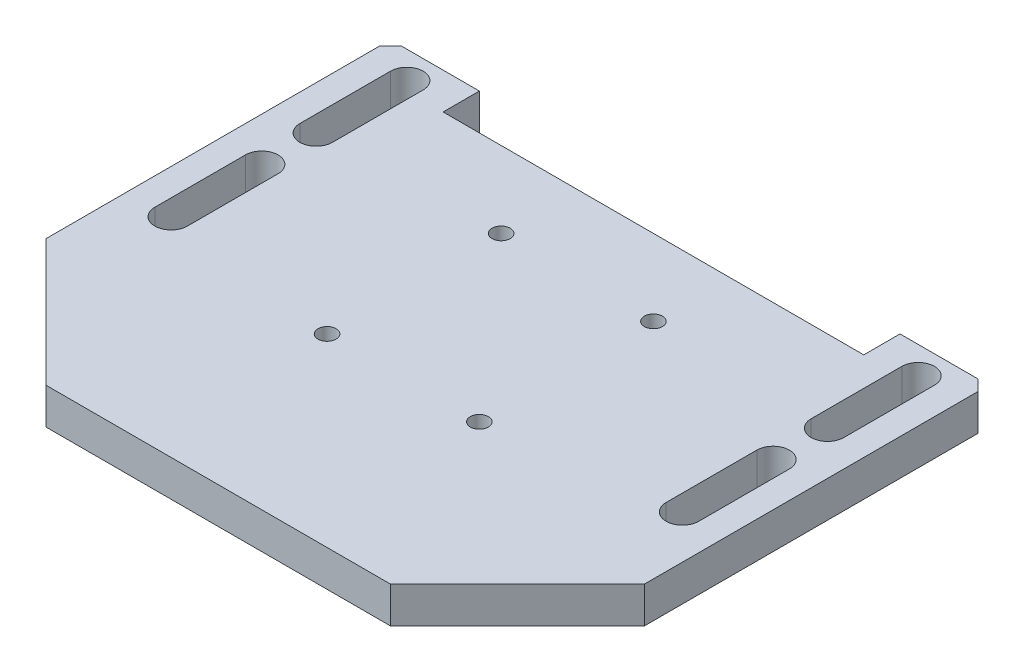
SolidWorks part; units mm, degrees
ref_plane "前视基准面" through (0, 0, 0) normal (0, 0, 1) x (1, 0, 0)
ref_plane "上视基准面" through (0, 0, 0) normal (0, 1, 0) x (1, 0, 0)
ref_plane "右视基准面" through (0, 0, 0) normal (1, 0, 0) x (0, 0, -1)
sketch "草图2" plane through (0, 0, 0) normal (0, 1, 0) x (1, 0, 0)
  line L1 (-82.5, 65) -> (82.5, 65)
  line L2 (-82.5, 65) -> (-82.5, -65)
  line L3 (-82.5, -65) -> (82.5, -65)
  line L4 (82.5, 65) -> (82.5, -65)
  line L5 (-82.5, 65) -> (82.5, -65) construction
  line L6 (-82.5, -65) -> (82.5, 65) construction
  point P0 (0, 0)
  dimension "D1" = 165
  dimension "D2" = 130
extrude "凸台-拉伸1" add sketch "草图2" along normal blind 10
sketch "草图3" plane through (0, 10, 0) normal (0, 1, 0) x (1, 0, 0)
  line L0 (82.5, 65) -> (-82.5, 65) construction
  line L1 (-58, 65) -> (58, 65)
  line L2 (-58, 65) -> (-58, 55)
  line L3 (-58, 55) -> (58, 55)
  line L4 (58, 65) -> (58, 55)
  line L5 (0, 0) -> (0, 72.8477) construction
  dimension "D1" = 116
  dimension "D2" = 10
extrude "切除-拉伸1" cut sketch "草图3" against normal blind 10
sketch "草图4" plane through (0, 10, 0) normal (0, 1, 0) x (1, 0, 0)
  line L0 (70.5, 57.5) -> (70.5, 32.5) construction
  line L1 (75, 57.5) -> (75, 32.5)
  line L2 (66, 57.5) -> (66, 32.5)
  line L3 (82.5, 65) -> (58, 65) construction
  line L4 (82.5, -65) -> (82.5, 65) construction
  line L5 (70.5, 17.5) -> (70.5, -7.5) construction
  line L6 (75, 17.5) -> (75, -7.5)
  line L7 (66, 17.5) -> (66, -7.5)
  line L14 (0, 0) -> (0, 80.0549) construction
  arc A0 (75, 57.5) -> (66, 57.5) centre (70.5, 57.5) ccw
  arc A1 (66, 32.5) -> (75, 32.5) centre (70.5, 32.5) ccw
  arc A2 (75, 17.5) -> (66, 17.5) centre (70.5, 17.5) ccw
  arc A3 (66, -7.5) -> (75, -7.5) centre (70.5, -7.5) ccw
  point P2 (70.5, 45)
  point P15 (70.5, 5)
  dimension "D1" = 25
  dimension "D2" = 9
  dimension "D3" = 20
  dimension "D4" = 12
  dimension "D6" = 40
  dimension "D5" = 2
extrude "切除-拉伸2" cut sketch "草图4" against normal through all
chamfer "倒角1" distance 35 angle 45 2 edges at (82.5, 5, 65) (-82.5, 5, 65)
chamfer "倒角2" [suppressed] distance 5 angle 45
hole_wizard "M6 螺纹孔1" positions "草图12" profile "草图11" tap size "M6" standard "ISO" end condition through all
sketch "草图12" plane through (0, 10, 0) normal (0, 1, 0) x (1, 0, 0)
  line L1 (0, 0) -> (0, -75.9524) construction
  point P0 (21, -14)
  point P2 (21, 34)
  point P12 (-21, 34)
  point P13 (-21, -14)
sketch "草图11" plane through (21, 10, 14) normal (1, 0, 0) x (0, 0, 1)
  line L0 (0, 0) -> (0, 10)
  line L1 (0, 10) -> (2.5, 10)
  line L2 (2.5, 10) -> (2.5, 0)
  line L5 (2.5, 0) -> (0, 0)
  line L11 (0, -6.35) -> (0, 107.95) construction
  dimension "通孔螺纹孔钻头直径" = 5
  dimension "通孔螺纹孔钻头深度" = 10
cosmetic thread "孔螺蚊线5" parameters "D2"=6
cosmetic thread "孔螺蚊线8" parameters "D2"=6
cosmetic thread "孔螺蚊线9" parameters "D2"=6
cosmetic thread "孔螺蚊线10" parameters "D2"=6
chamfer "倒角3" distance 3 angle 45 2 edges at (82.5, 5, -65) (-82.5, 5, -65)
mirror "镜向1" about plane through (0, 0, 0) normal (1, 0, 0) of "切除-拉伸2"
